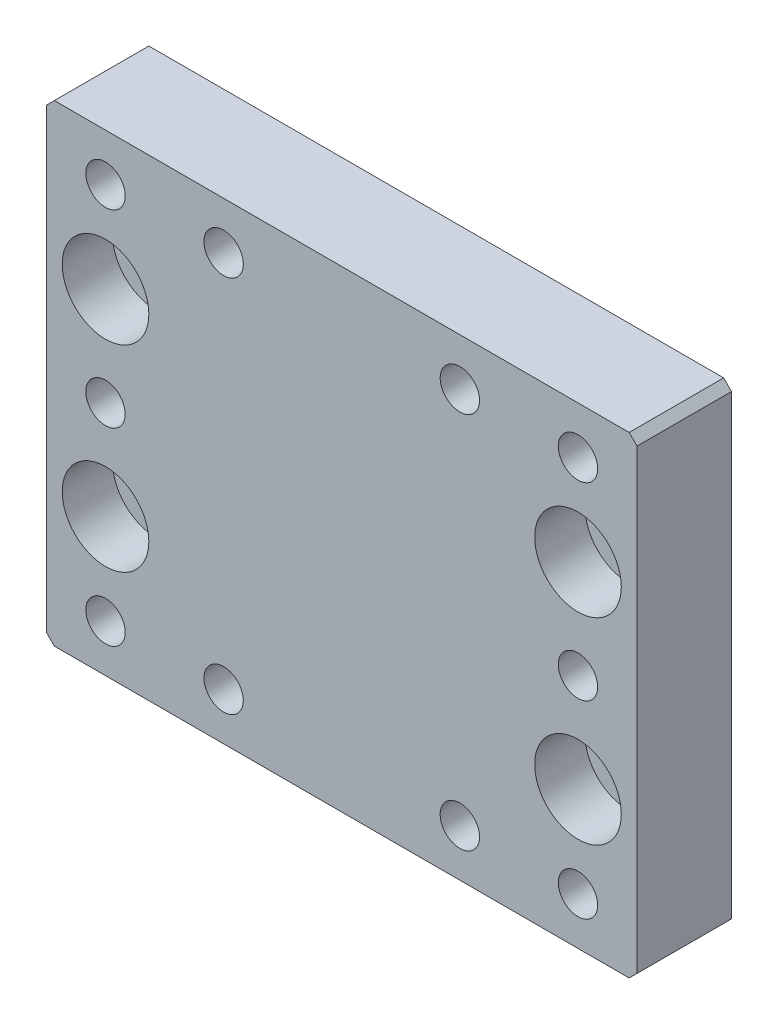
from build123d import *

# Parameters (mm, degrees)
SKETCH1_W                                           = 75
SKETCH1_H                                           = 60
BOSS_EXTRUDE1_DEPTH                                 = 6
M6_TAPPED_HOLE1_D                                   = 5
CBORE_FOR_M6_HEX_SOCKET_HEAD_CAP_SCREW1_D           = 6.6
CBORE_FOR_M6_HEX_SOCKET_HEAD_CAP_SCREW1_CBORE_D     = 11
CBORE_FOR_M6_HEX_SOCKET_HEAD_CAP_SCREW1_CBORE_DEPTH = 6.4
BLIND_PIN_HOLE3_SIZE_MM_D                           = 5
BLIND_PIN_HOLE3_SIZE_MM_DEPTH                       = 11
BLIND_PIN_HOLE3_SIZE_MM_TIP                         = 1.502151548
MM_3_D                                              = 5
MM_3_DEPTH                                          = 10
MM_3_TIP                                            = 1.502151548
CHAMFER1_SIZE                                       = 1


with BuildPart() as part:
    # Sketch1 → Boss-Extrude1 (new, symmetric)
    with BuildSketch(Plane.XY):
        Rectangle(SKETCH1_W, SKETCH1_H)
    extrude(amount=BOSS_EXTRUDE1_DEPTH, both=True)

    # M6 Tapped Hole1 (through all)
    with Locations(Plane.XY.offset(6)):
        with Locations((30, 24), (30, -24), (-30, -24), (-30, 24)):
            Hole(M6_TAPPED_HOLE1_D / 2)

    # CBORE for M6 Hex Socket Head Cap Screw1 (through all)
    with Locations(Plane.XY.offset(6)):
        with Locations((-30, 12.5), (30, 12.5), (-30, -12.5), (30, -12.5)):
            CounterBoreHole(CBORE_FOR_M6_HEX_SOCKET_HEAD_CAP_SCREW1_D / 2, CBORE_FOR_M6_HEX_SOCKET_HEAD_CAP_SCREW1_CBORE_D / 2, CBORE_FOR_M6_HEX_SOCKET_HEAD_CAP_SCREW1_CBORE_DEPTH)

    # Blind Pin Hole3 (size mm)
    with Locations(Plane.XY.offset(6)):
        with Locations((-30, 0), (30, 0)):
            Hole(BLIND_PIN_HOLE3_SIZE_MM_D / 2, depth=BLIND_PIN_HOLE3_SIZE_MM_DEPTH)
            with Locations((0, 0, -(BLIND_PIN_HOLE3_SIZE_MM_DEPTH + BLIND_PIN_HOLE3_SIZE_MM_TIP / 2))):  # 118° drill point
                Cone(0, BLIND_PIN_HOLE3_SIZE_MM_D / 2, BLIND_PIN_HOLE3_SIZE_MM_TIP, mode=Mode.SUBTRACT)

    # 大小mm 暗销孔3
    with Locations(Plane.XY.offset(6)):
        with Locations((-15, 24), (15, -24), (15, 24), (-15, -24)):
            Hole(MM_3_D / 2, depth=MM_3_DEPTH)
            with Locations((0, 0, -(MM_3_DEPTH + MM_3_TIP / 2))):  # 118° drill point
                Cone(0, MM_3_D / 2, MM_3_TIP, mode=Mode.SUBTRACT)

    # Chamfer1
    chamfer1_edges = [part.edges().sort_by_distance(p)[0] for p in [
        (37.5, -30, 0),
        (-37.5, -30, 0),
        (-37.5, 30, 0),
        (37.5, 30, 0),
    ]]
    chamfer(chamfer1_edges, length=CHAMFER1_SIZE)


solid = part.part
